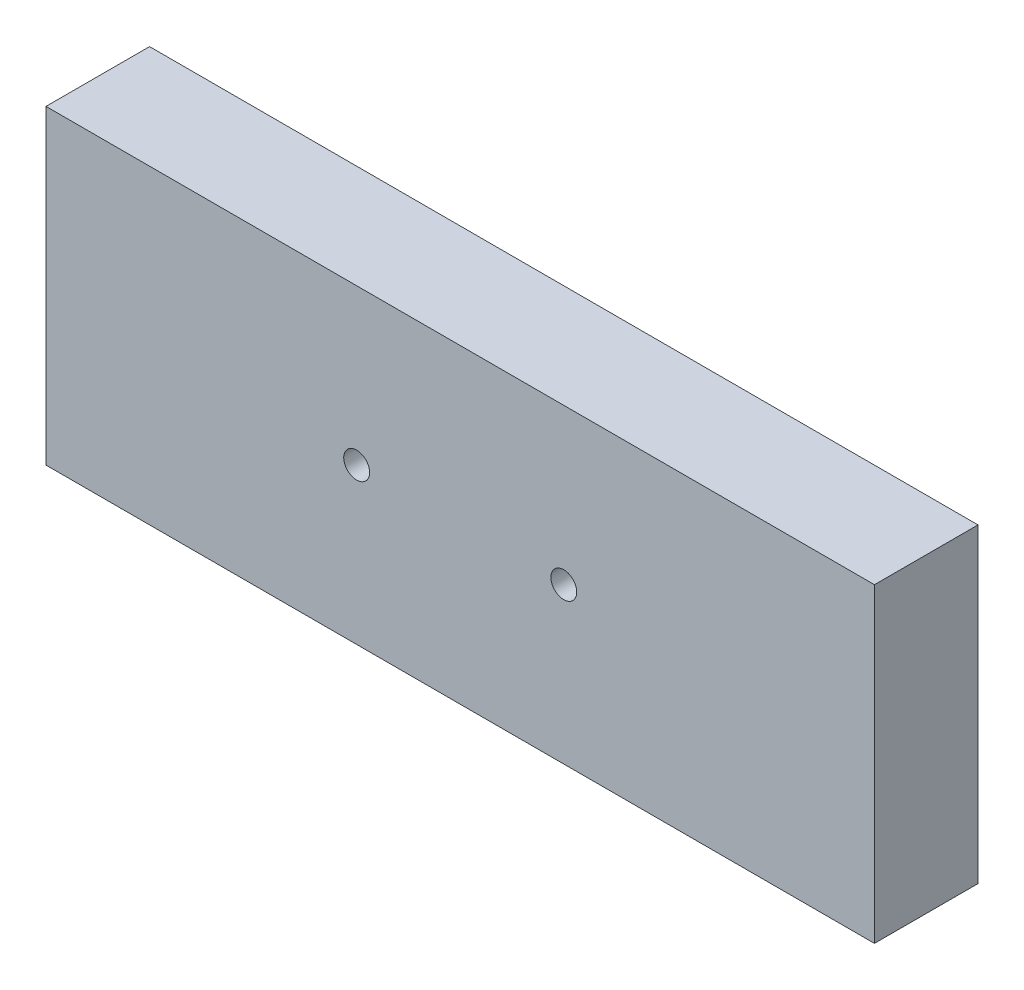
from build123d import *

# Parameters (mm, degrees)
SKETCH_1_W          = 80
SKETCH_1_H          = 30
EXTRUDE_1_DEPTH     = 10
SKETCH_2_R          = 1.25
CUT_EXTRUDE_1_DEPTH = 2


with BuildPart() as part:
    # 草图1 → 凸台-拉伸1 (new body)
    with BuildSketch(Plane.XY):
        Rectangle(SKETCH_1_W, SKETCH_1_H)
    extrude(amount=EXTRUDE_1_DEPTH)

    # 草图2 → 切除-拉伸1 (cut)
    with BuildSketch(Plane.XY.offset(10)):
        with Locations((-10, 0)):
            Circle(SKETCH_2_R)
        with Locations((10, 0)):
            Circle(SKETCH_2_R)
    extrude(amount=-CUT_EXTRUDE_1_DEPTH, mode=Mode.SUBTRACT)


solid = part.part
